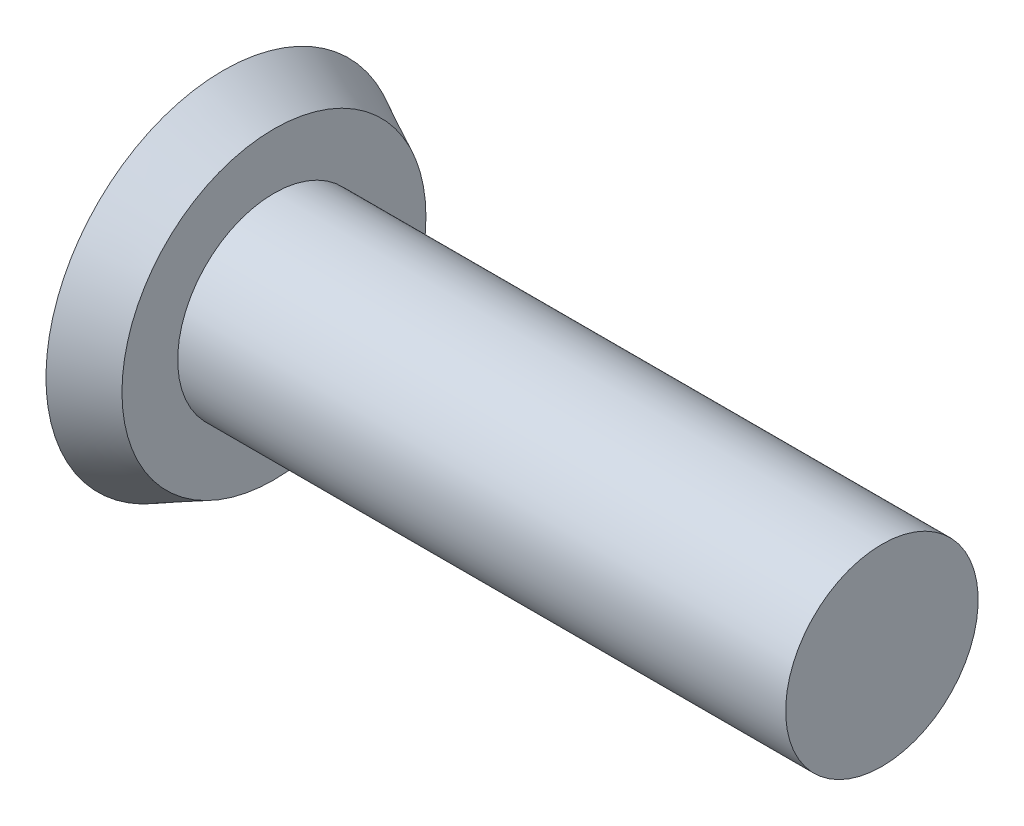
from build123d import *


with BuildPart() as part:
    # Sketch1 → Revolve1 (revolve)
    with BuildSketch(Plane.XY):
        Polygon((0, 0), (0, 3.5), (1, 3), (1, 1.9), (13, 1.9), (13, 0), align=None)
    revolve(axis=Axis((13, 0, 0), (-1, 0, 0)))


solid = part.part
